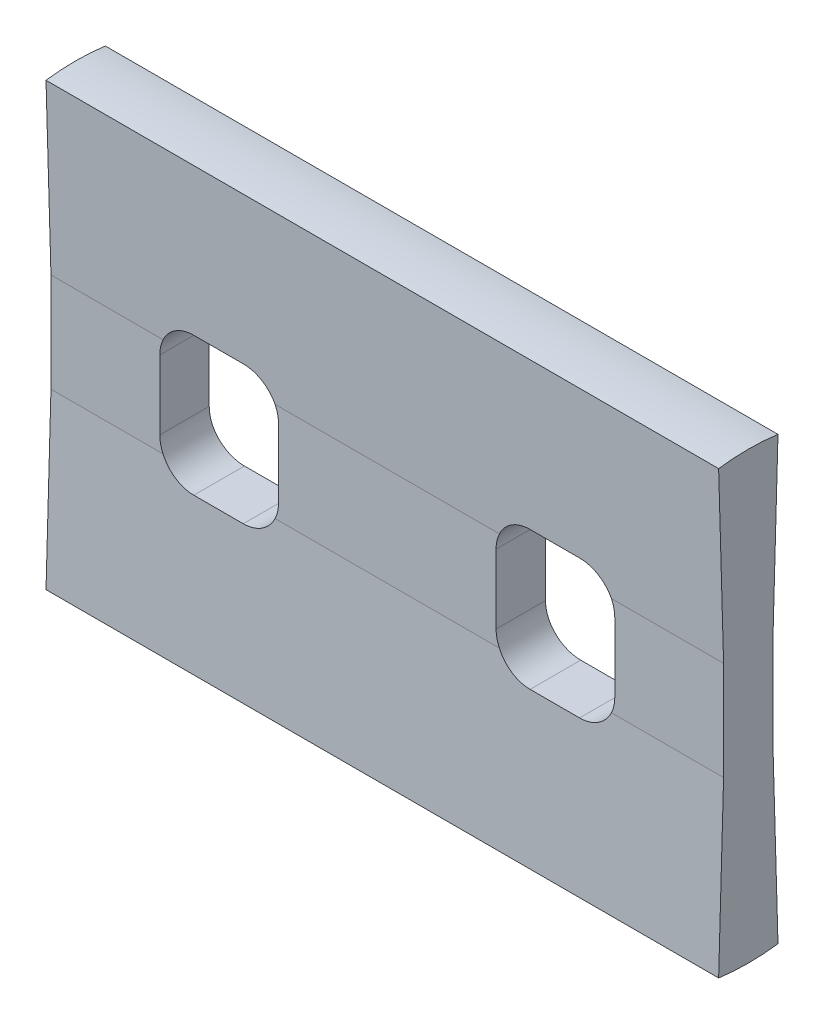
from build123d import *

# Parameters (mm, degrees)
BOSS_EXTRUDE1_DEPTH = 340
CUT_EXTRUDE1_DEPTH  = 409.809246471


with BuildPart() as part:
    # Sketch1 → Boss-Extrude1 (new, symmetric)
    with BuildSketch(Plane(origin=(0, 0, 0), x_dir=(0, 0, -1), z_dir=(1, 0, 0))):
        with BuildLine():
            Line((25, -50), (25, 50))
            Line((25, 50), (30, 222.99103121))
            ThreePointArc((30, 222.99103121), (0, 225), (-30, 222.99103121))
            Line((-30, 222.99103121), (-25, 50))
            Line((-25, 50), (-25, -50))
            Line((-25, -50), (-30, -222.99103121))
            ThreePointArc((-30, -222.99103121), (0, -225), (30, -222.99103121))
            Line((30, -222.99103121), (25, -50))
        make_face()
    extrude(amount=BOSS_EXTRUDE1_DEPTH, both=True)

    # Sketch2 → Cut-Extrude1 (cut, symmetric)
    with BuildSketch(Plane.XY):
        with BuildLine():
            Line((-145, -70), (-195, -70))
            ThreePointArc((-195, -70), (-219.748737342, -59.748737342), (-230, -35))
            Line((-230, -35), (-230, 35))
            ThreePointArc((-230, 35), (-219.748737342, 59.748737342), (-195, 70))
            Line((-195, 70), (-145, 70))
            ThreePointArc((-145, 70), (-120.251262658, 59.748737342), (-110, 35))
            Line((-110, 35), (-110, -35))
            ThreePointArc((-110, -35), (-120.251262658, -59.748737342), (-145, -70))
        make_face()
    cut_extrude1 = extrude(amount=CUT_EXTRUDE1_DEPTH, both=True, mode=Mode.SUBTRACT)

    # Mirror1: Cut-Extrude1 across plane
    add(cut_extrude1.mirror(Plane(origin=(0, 0, 0), x_dir=(0, 0, 1), z_dir=(1, 0, 0))), mode=Mode.SUBTRACT)


solid = part.part
